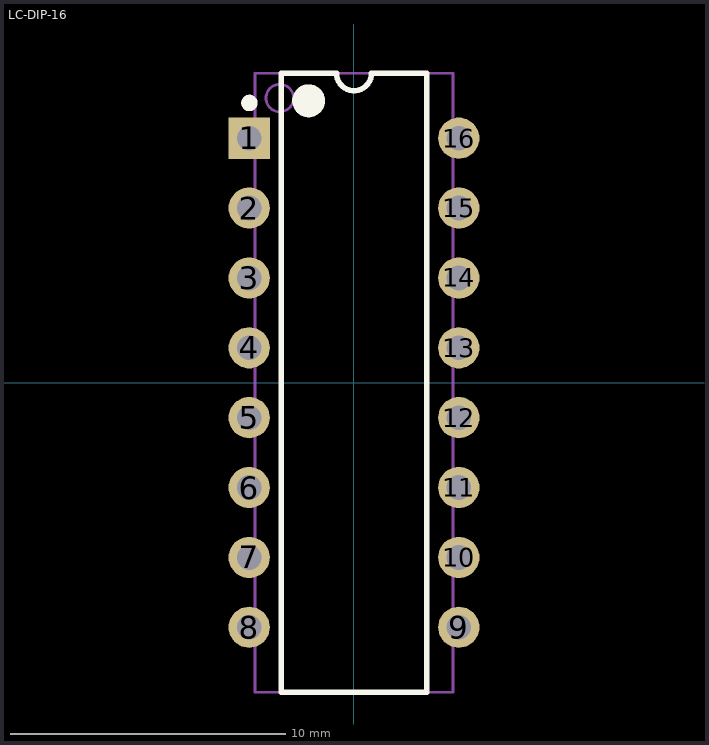
[diagram p0: the footprint, top view; thin cyan lines are the x and y axes]
# Altium footprint library MISC86340-8.PcbLib: 1 footprints
Each footprint in its own frame and in the unit in brackets; x right, y up, seen from the top. Pads: shape width x height; smd on the part's side, far side on the other; paste and mask are expansions set on the pad; w line width, h text height; cw(c..) or ccw(c..) is an arc to the next point about the centre after c.

## LC-DIP-16 [mm]
pads (16):
  rect 1.5x1.5 hole 0.9: 1(-3.81,8.89)
  round 1.5 hole 0.9: 2(-3.81,6.35) 3(-3.81,3.81) 4(-3.81,1.27) 5(-3.81,-1.27) 6(-3.81,-3.81) 7(-3.81,-6.35) 8(-3.81,-8.89) 9(3.81,-8.89) 10(3.81,-6.35) 11(3.81,-3.81) 12(3.81,-1.27) 13(3.81,1.27) 14(3.81,3.81) 15(3.81,6.35) 16(3.81,8.89)
Top Overlay:
  circle w0.3: c-3.8,10.17 r0.15
  circle w0.6: c-1.65,10.25 r0.3
  lines w0.2: -2.65,-11.25 -2.65,11.25 -0.635,11.25 ccw(c0,11.25) 0.635,11.25 2.65,11.25 2.65,-11.25 -2.65,-11.25
Mechanical 13:
  circle w0.1: c-2.7,10.35 r0.5
  lines w0.1: -3.6,-11.25 -3.6,11.25 3.6,11.25 3.6,-11.25 -3.6,-11.25